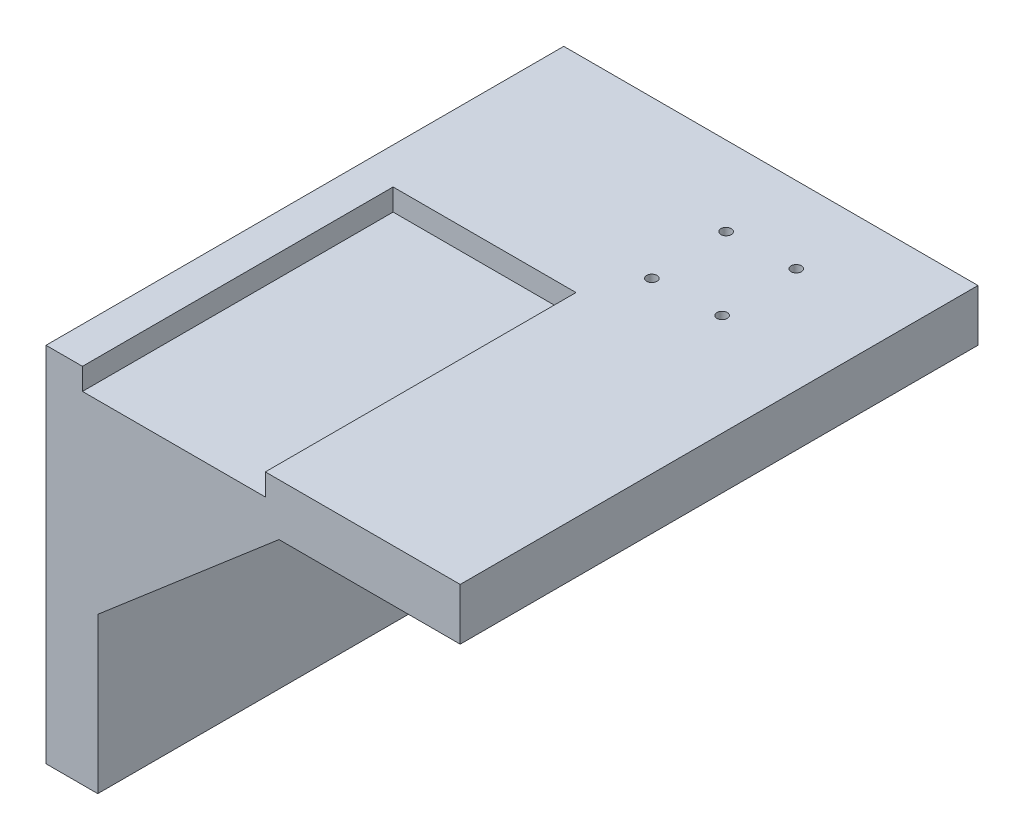
SolidWorks part; units mm, degrees
material "1023 碳钢板 (SS)"
ref_plane "前视基准面" through (0, 0, 0) normal (0, 0, 1) x (1, 0, 0)
ref_plane "上视基准面" through (0, 0, 0) normal (0, 1, 0) x (1, 0, 0)
ref_plane "右视基准面" through (0, 0, 0) normal (1, 0, 0) x (0, 0, -1)
sketch "草图1" plane through (0, 0, 0) normal (0, 0, 1) x (1, 0, 0)
  line L0 (-37.5, 32.7885) -> (42.5, 32.7885)
  line L1 (42.5, 32.7885) -> (42.5, 22.7885)
  line L2 (42.5, 22.7885) -> (-27.5, 22.7885)
  line L3 (-27.5, 22.7885) -> (-27.5, -37.2115)
  line L4 (-27.5, -37.2115) -> (-37.5, -37.2115)
  line L5 (-37.5, -37.2115) -> (-37.5, 32.7885)
  dimension "D1" = 10
  dimension "D2" = 10
  dimension "D3" = 70
  dimension "D4" = 60
extrude "凸台-拉伸1" add sketch "草图1" along normal blind 100
sketch "草图2" plane through (0, 0, 100) normal (0, 0, 1) x (1, 0, 0)
  line L0 (-30.458, 32.7885) -> (-30.458, 28.5885)
  line L1 (42.5, 32.7885) -> (-37.5, 32.7885) construction
  line L2 (-30.458, 28.5885) -> (4.8599, 28.5885)
  line L3 (4.8599, 28.5885) -> (4.8599, 32.7885)
  line L4 (4.8599, 32.7885) -> (-30.458, 32.7885)
  dimension "D1" = 4.2
extrude "切除-拉伸1" cut sketch "草图2" against normal blind 60
ref_plane "基准面1" through (0, 0, 95) normal (0, 0, 1) x (1, 0, 0)
sketch "草图5" plane through (0, 0, 95) normal (0, 0, 1) x (1, 0, 0)
  line L0 (7.5, 22.7885) -> (-27.5, -7.2115)
  line L1 (-27.5, 22.7885) -> (42.5, 22.7885) construction
  line L2 (-27.5, -37.2115) -> (-27.5, 22.7885) construction
rib "筋6" sketch "草图5" sketch "草图5" thickness 10 extrusion direction parallel to sketch draft on no parameters "D1"=10
extrude "切除-拉伸2" cut sketch "草图6" against normal up to surface (10 mm away) up to face at (-37.5, -2.2115, 50)
sketch "草图6" plane through (-27.5, 891.5327, -866.3577) normal (1, 0, 0) x (0, 0, 1)
  circle A2 centre (900.2498, 880.97) radius 3
  circle A3 centre (890.7128, 880.97) radius 3
  circle A4 centre (900.2498, 913.1376) radius 3
  circle A5 centre (890.7128, 913.1376) radius 3
extrude "切除-拉伸3" cut sketch "草图7" against normal blind 15
sketch "草图7" plane through (1081.4559, 22.7885, -866.3577) normal (0, -1, 0) x (-0.0785, 0, 0.9969)
  line L0 (957.1306, 1000.5442) -> (983.9293, 997.2537) construction
  line L3 (955.5463, 987.6411) -> (982.345, 984.3506) construction
  circle A0 centre (963.0859, 999.813) radius 1
  circle A1 centre (977.9741, 997.9849) radius 1
  circle A2 centre (961.5016, 986.9099) radius 1
  circle A3 centre (976.3898, 985.0818) radius 1
sketch "草图8" plane through (0, 32.7885, 0) normal (0, 1, 0) x (1, 0, 0)
  circle A0 centre (9.1622, -15.3149) radius 1
  circle A1 centre (9.8165, -30.3006) radius 1
  circle A2 centre (22.8041, -29.7335) radius 1
  circle A3 centre (22.1498, -14.7478) radius 1
sketch "草图9" plane through (-37.5, 0, 0) normal (-1, 0, 0) x (0, 0, 1)
  circle A0 centre (24.3551, 10.5627) radius 3
  circle A1 centre (33.8921, 10.5627) radius 3
  circle A2 centre (24.3551, -21.6049) radius 3
  circle A3 centre (33.8921, -21.6049) radius 3
